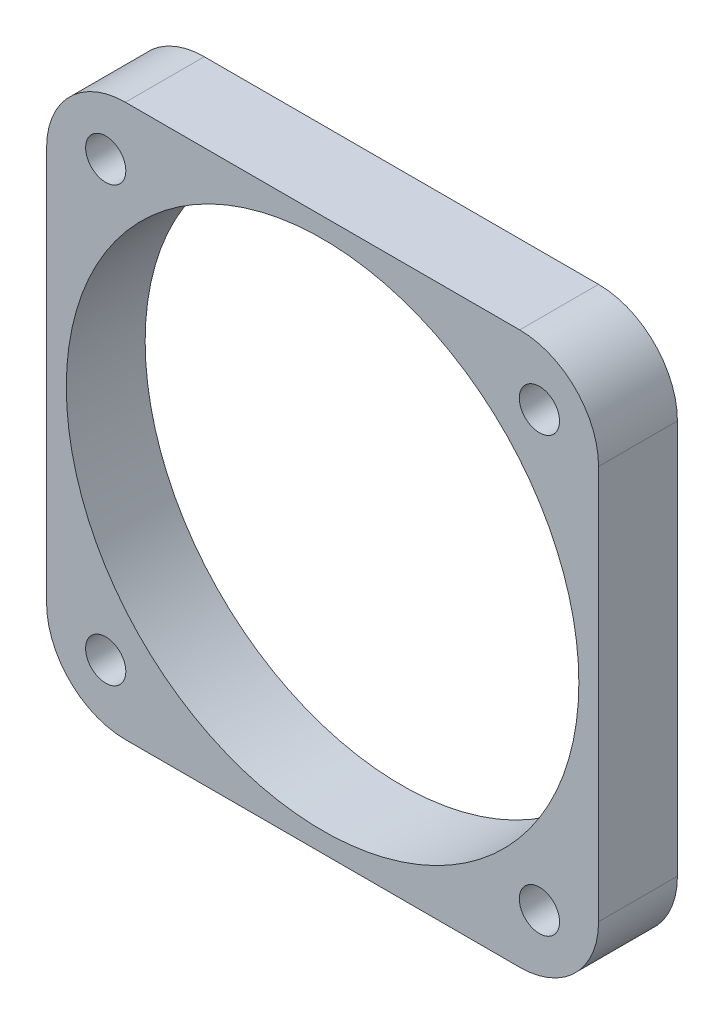
SolidWorks part; units mm, degrees
ref_plane "Front Plane" through (0, 0, 0) normal (0, 0, 1) x (1, 0, 0)
ref_plane "Top Plane" through (0, 0, 0) normal (0, 1, 0) x (1, 0, 0)
ref_plane "Right Plane" through (0, 0, 0) normal (1, 0, 0) x (0, 0, -1)
sketch "Sketch1" plane through (0, 0, 0) normal (0, 0, 1) x (1, 0, 0)
  line L1 (20, 0) -> (120, 0)
  line L2 (0, 20) -> (0, 120)
  line L3 (20, 140) -> (120, 140)
  line L4 (140, 20) -> (140, 120)
  circle A0 centre (70, 70) radius 65
  arc A1 (20, 0) -> (0, 20) centre (20, 20) cw
  arc A2 (120, 0) -> (140, 20) centre (120, 20) ccw
  arc A3 (120, 140) -> (140, 120) centre (120, 120) cw
  arc A4 (0, 120) -> (20, 140) centre (20, 120) cw
  point P9 (0, 0)
  point P14 (140, 140)
  point P17 (0, 140)
  dimension "D3" = 20
  dimension "D1" = 140
  dimension "D2" = 140
extrude "Boss-Extrude1" add sketch "Sketch1" along normal blind 20
sketch "Sketch2" plane through (0, 0, 20) normal (0, 0, 1) x (1, 0, 0)
  circle A1 centre (15, 125) radius 5.9
  circle A2 centre (125, 125) radius 5.9
  circle A3 centre (125, 15) radius 5.9
  circle A4 centre (15, 15) radius 5.9
hole_wizard "M12 Tapped Hole1" positions "3DSketch1" profile "Sketch3" tap size "M12" standard "Gb"
sketch3d "3DSketch1"
  point P0 (15, 125, 20)
  point P3 (125, 125, 20)
  point P6 (125, 15, 20)
  point P9 (15, 15, 20)
sketch "Sketch3" plane through (15, 125, 20) normal (1, 0, 0) x (0, -1, 0)
  line L0 (0, 0) -> (0, 19.0644)
  line L1 (0, 19.0644) -> (5.1, 16)
  line L2 (5.1, 16) -> (5.1, 0)
  line L5 (5.1, 0) -> (0, 0)
  line L10 (0, 19.0644) -> (-5.1, 16) construction
  line L11 (0, -6.35) -> (0, 107.95) construction
  dimension "螺纹孔钻头直径" = 10.2
  dimension "螺纹孔钻头深度" = 16
  dimension "导头角度" = 118
cosmetic thread "Cosmetic Thread1" parameters "D1"=12, "D2"=12
cosmetic thread "Cosmetic Thread2" parameters "D1"=12, "D2"=12
cosmetic thread "Cosmetic Thread3" parameters "D1"=12, "D2"=12
cosmetic thread "Cosmetic Thread4" parameters "D1"=12, "D2"=12
